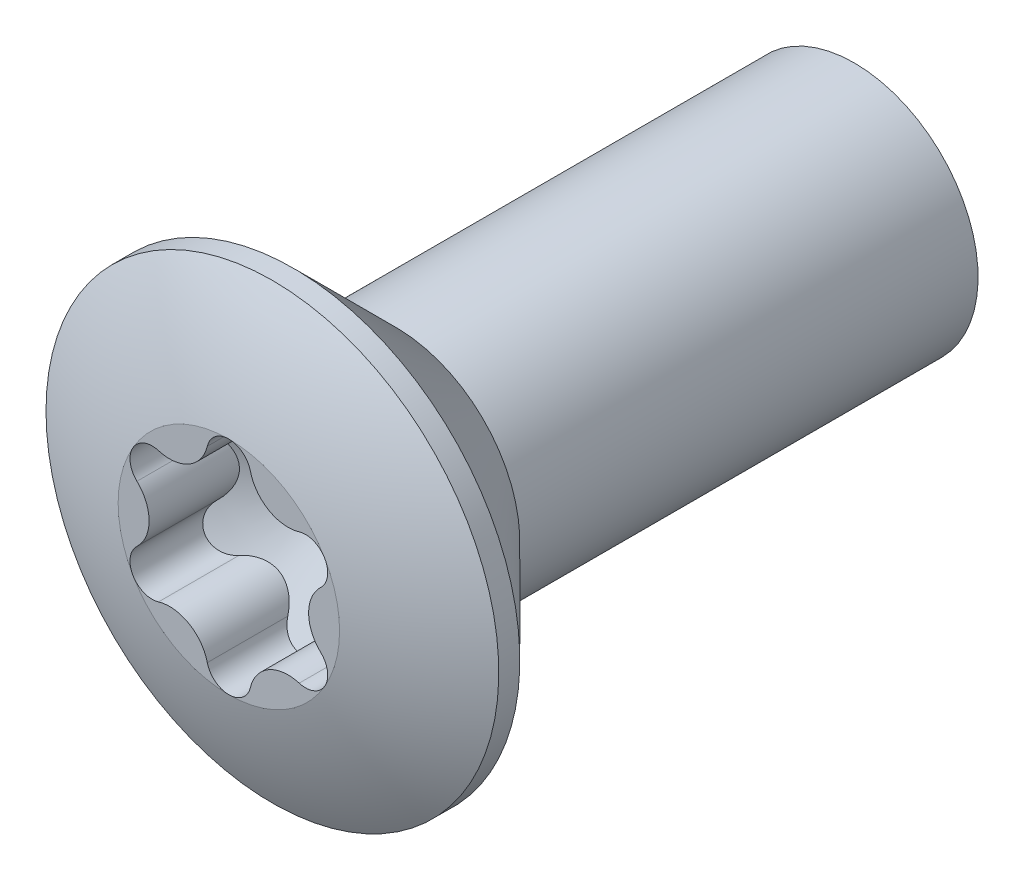
from build123d import *

# Parameters (mm, degrees)
HEXALOBULAR_REACH = 30.827


with BuildPart() as part:
    # BodySke → Base-Revolve (revolve)
    with BuildSketch(Plane(origin=(0, 0, 0), x_dir=(0, 0, -1), z_dir=(1, 0, 0)), mode=Mode.PRIVATE) as base_revolve_sk:
        with BuildLine():
            Line((3.130026132, 9.15), (7.280026132, 5))
            Line((7.280026132, 5), (26.280026132, 5))
            Line((26.280026132, 5), (26.280026132, 0))
            Line((26.280026132, 0), (0, 0))
            ThreePointArc((0, 0), (0.578590295, 4.714897114), (2.280026132, 9.15))
            Line((2.280026132, 9.15), (3.130026132, 9.15))
        make_face()
    revolve(base_revolve_sk.sketch.rotate(Axis((0, 0, 0), (0, 0, 1)), 90), axis=Axis((0, 0, 0), (0, 0, 1)))

    # PreBSke → PreBroach (revolve, cut)
    with BuildSketch(Plane(origin=(0, 0, 0), x_dir=(0, 0, -1), z_dir=(1, 0, 0))):
        Polygon((0, 0), (0, 4.475), (3.42, 4.475), (6.10885127, 0), align=None)
    revolve(axis=Axis((0, 0, 0), (0, 0, 1)), mode=Mode.SUBTRACT)

    # Hexalobular: up to this cone (the profile starts inside it)
    hexalobular_end = Plane(origin=(0, 0, -0.520422), z_dir=(0, 0, 1)).offset(-5.58842827) * Cone(1.664e-06, 76.9165693, 46.216136443, align=(Align.CENTER, Align.CENTER, Align.MIN), mode=Mode.PRIVATE)
    # HexSke → Hexalobular (add, up to the surface)
    with BuildSketch(Plane.XY.offset(-0.52042216), mode=Mode.PRIVATE) as hexalobular_sk1:
        with BuildLine():
            ThreePointArc((-3.875463682, -2.2375), (-3.985930746, -1.660351093), (-3.714652929, -1.139090909))
            ThreePointArc((-3.714652929, -1.139090909), (-3.2233964, 0), (-3.714652929, 1.139090909))
            ThreePointArc((-3.714652929, 1.139090909), (-3.985930746, 1.660351093), (-3.875463682, 2.2375))
            ThreePointArc((-3.875463682, 2.2375), (-4.475, 0), (-3.875463682, -2.2375))
        make_face()
    hexalobular_tool1 = extrude(hexalobular_sk1.sketch, amount=-HEXALOBULAR_REACH, mode=Mode.PRIVATE) & hexalobular_end
    add(hexalobular_tool1.solids().sort_by_distance((-3.918157, 0, -0.520422))[0])
    # HexSke → Hexalobular (add, up to the surface)
    with BuildSketch(Plane.XY.offset(-0.52042216), mode=Mode.PRIVATE) as hexalobular_sk2:
        with BuildLine():
            ThreePointArc((-2.843808129, -2.647438348), (-3.430871599, -2.621741738), (-3.875463682, -2.2375))
            ThreePointArc((-3.875463682, -2.2375), (-2.2375, -3.875463682), (0, -4.475))
            ThreePointArc((0, -4.475), (-0.555059148, -4.282092831), (-0.8708448, -3.786529257))
            ThreePointArc((-0.8708448, -3.786529257), (-1.6116982, -2.791543169), (-2.843808129, -2.647438348))
        make_face()
    hexalobular_tool2 = extrude(hexalobular_sk2.sketch, amount=-HEXALOBULAR_REACH, mode=Mode.PRIVATE) & hexalobular_end
    add(hexalobular_tool2.solids().sort_by_distance((-1.959079, -3.393224, -0.520422))[0])
    # HexSke → Hexalobular (add, up to the surface)
    with BuildSketch(Plane.XY.offset(-0.52042216), mode=Mode.PRIVATE) as hexalobular_sk3:
        with BuildLine():
            ThreePointArc((0, 4.475), (-2.2375, 3.875463682), (-3.875463682, 2.2375))
            ThreePointArc((-3.875463682, 2.2375), (-3.430871599, 2.621741738), (-2.843808129, 2.647438348))
            ThreePointArc((-2.843808129, 2.647438348), (-1.6116982, 2.791543169), (-0.8708448, 3.786529257))
            ThreePointArc((-0.8708448, 3.786529257), (-0.555059148, 4.282092831), (0, 4.475))
        make_face()
    hexalobular_tool3 = extrude(hexalobular_sk3.sketch, amount=-HEXALOBULAR_REACH, mode=Mode.PRIVATE) & hexalobular_end
    add(hexalobular_tool3.solids().sort_by_distance((-1.959079, 3.393224, -0.520422))[0])
    # HexSke → Hexalobular (add, up to the surface)
    with BuildSketch(Plane.XY.offset(-0.52042216), mode=Mode.PRIVATE) as hexalobular_sk4:
        with BuildLine():
            ThreePointArc((0.8708448, -3.786529257), (0.555059148, -4.282092831), (0, -4.475))
            ThreePointArc((0, -4.475), (2.2375, -3.875463682), (3.875463682, -2.2375))
            ThreePointArc((3.875463682, -2.2375), (3.430871599, -2.621741738), (2.843808129, -2.647438348))
            ThreePointArc((2.843808129, -2.647438348), (1.6116982, -2.791543169), (0.8708448, -3.786529257))
        make_face()
    hexalobular_tool4 = extrude(hexalobular_sk4.sketch, amount=-HEXALOBULAR_REACH, mode=Mode.PRIVATE) & hexalobular_end
    add(hexalobular_tool4.solids().sort_by_distance((1.959079, -3.393224, -0.520422))[0])
    # HexSke → Hexalobular (add, up to the surface)
    with BuildSketch(Plane.XY.offset(-0.52042216), mode=Mode.PRIVATE) as hexalobular_sk5:
        with BuildLine():
            ThreePointArc((3.875463682, 2.2375), (2.2375, 3.875463682), (0, 4.475))
            ThreePointArc((0, 4.475), (0.555059148, 4.282092831), (0.8708448, 3.786529257))
            ThreePointArc((0.8708448, 3.786529257), (1.6116982, 2.791543169), (2.843808129, 2.647438348))
            ThreePointArc((2.843808129, 2.647438348), (3.430871599, 2.621741738), (3.875463682, 2.2375))
        make_face()
    hexalobular_tool5 = extrude(hexalobular_sk5.sketch, amount=-HEXALOBULAR_REACH, mode=Mode.PRIVATE) & hexalobular_end
    add(hexalobular_tool5.solids().sort_by_distance((1.959079, 3.393224, -0.520422))[0])
    # HexSke → Hexalobular (add, up to the surface)
    with BuildSketch(Plane.XY.offset(-0.52042216), mode=Mode.PRIVATE) as hexalobular_sk6:
        with BuildLine():
            ThreePointArc((3.714652929, -1.139090909), (3.985930746, -1.660351093), (3.875463682, -2.2375))
            ThreePointArc((3.875463682, -2.2375), (4.475, 0), (3.875463682, 2.2375))
            ThreePointArc((3.875463682, 2.2375), (3.985930746, 1.660351093), (3.714652929, 1.139090909))
            ThreePointArc((3.714652929, 1.139090909), (3.2233964, 0), (3.714652929, -1.139090909))
        make_face()
    hexalobular_tool6 = extrude(hexalobular_sk6.sketch, amount=-HEXALOBULAR_REACH, mode=Mode.PRIVATE) & hexalobular_end
    add(hexalobular_tool6.solids().sort_by_distance((3.918157, 0, -0.520422))[0])

    # ThdSchSke → ThreadSchematic (revolve, cut)
    with BuildSketch(Plane(origin=(0, 0, 0), x_dir=(0, 0, -1), z_dir=(1, 0, 0))):
        Polygon((26.758072155, 5), (26.280026132, 4.172), (25.80198011, 5), align=None)
    revolve(axis=Axis((0, 0, 0), (0, 0, 1)), mode=Mode.SUBTRACT)


solid = part.part
